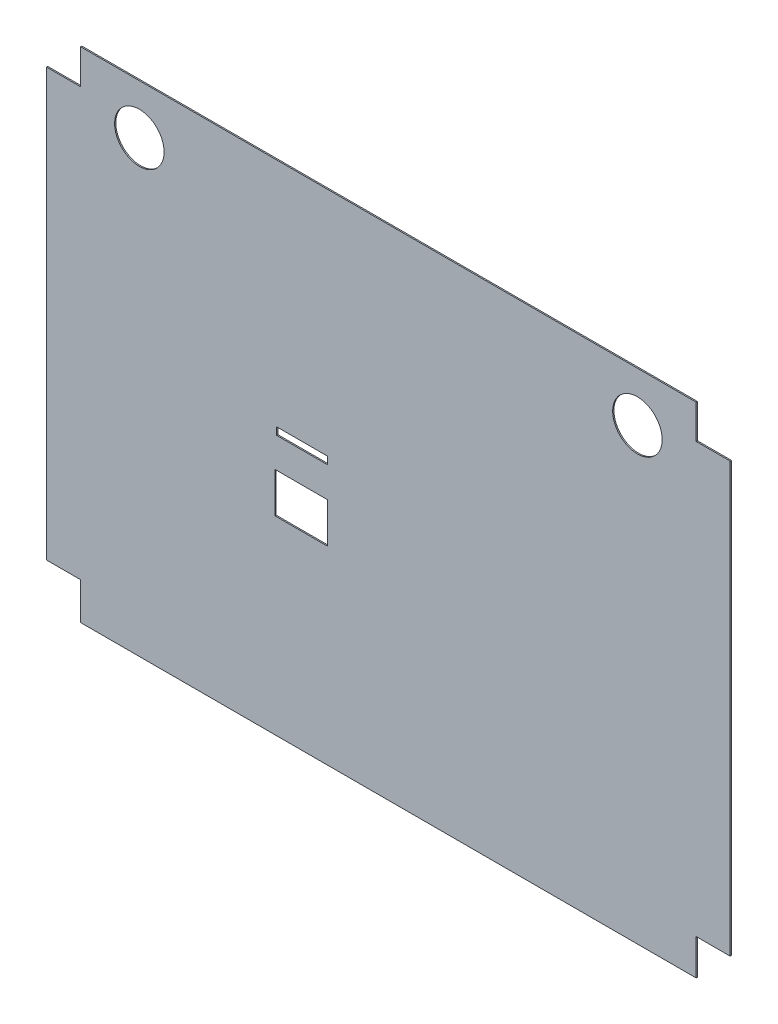
from build123d import *

# Parameters (mm, degrees)
SKETCH_1_R          = 40
EXTRUDE_1_DEPTH     = 2
SKETCH_3_W          = 12
SKETCH_3_H          = 82
CUT_EXTRUDE_2_DEPTH = 2
CUT_EXTRUDE_3_DEPTH = 2


with BuildPart() as part:
    # 草图1 → 凸台-拉伸1 (new body)
    with BuildSketch(Plane.XY):
        Polygon((-367.770666468, 104.233847936), (-312.770666468, 104.233847936), (-312.770666468, 160.233847936), (682.229333532, 160.233847936), (682.229333532, 105.233847936), (737.229333532, 105.233847936), (737.229333532, -587.766152064), (682.229333532, -587.766152064), (682.229333532, -645.766152064), (-312.770666468, -645.766152064), (-312.770666468, -585.766152064), (-367.770666468, -585.766152064), align=None)
        with Locations((-217.770666468, 80.233847936)):
            Circle(SKETCH_1_R, mode=Mode.SUBTRACT)
        with Locations((587.229333532, 80.233847936)):
            Circle(SKETCH_1_R, mode=Mode.SUBTRACT)
    extrude(amount=EXTRUDE_1_DEPTH)

    # 草图3 → 切除-拉伸2 (cut)
    with BuildSketch(Plane(origin=(995.435508438, 654.453268367, 0), x_dir=(0, -1, 0), z_dir=(0, 0, -1))):
        with Locations((873.744003867, 950.143932906)):
            Rectangle(SKETCH_3_W, SKETCH_3_H)
    extrude(amount=-CUT_EXTRUDE_2_DEPTH, mode=Mode.SUBTRACT)

    # 草图4 → 切除-拉伸3 (cut)
    with BuildSketch(Plane(origin=(995.435508438, 654.453268367, 0), x_dir=(0, -1, 0), z_dir=(0, 0, -1))):
        Polygon((928.744003867, 949.143932916), (928.744003867, 909.143932916), (993.744003867, 909.143932916), (993.744003867, 949.143932916), (993.744003867, 994.143932916), (928.744003867, 994.143932916), align=None)
    extrude(amount=-CUT_EXTRUDE_3_DEPTH, mode=Mode.SUBTRACT)


solid = part.part
